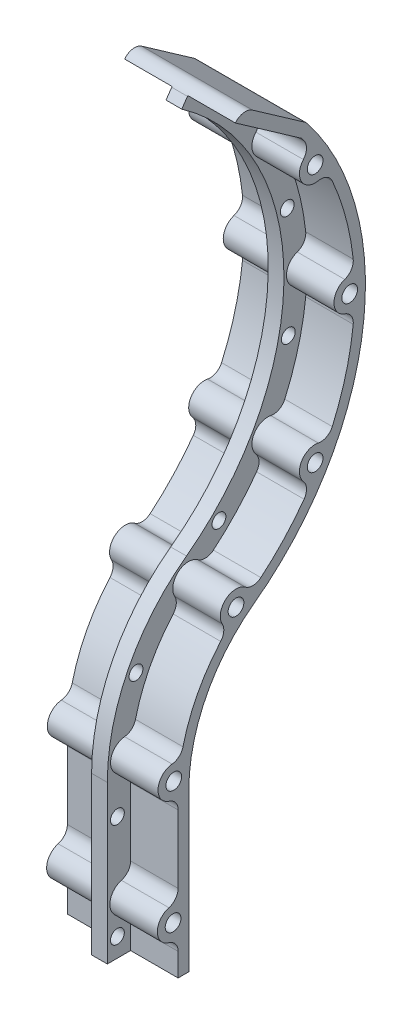
SolidWorks part; units mm, degrees
material "6061 合金"
ref_plane "前视基准面" through (0, 0, 0) normal (0, 0, 1) x (1, 0, 0)
ref_plane "上视基准面" through (0, 0, 0) normal (0, 1, 0) x (1, 0, 0)
ref_plane "右视基准面" through (0, 0, 0) normal (1, 0, 0) x (0, 0, -1)
sketch "弹链路径" plane through (0, 0, 0) normal (1, 0, 0) x (0, 0, -1)
  line L0 (0, -41.5) -> (0, 0)
  line L1 (0, 80) -> (6.1652, 79.4606)
  line L2 (0, 80) -> (3.3166, 80) construction
  arc A0 (18.3088, 36.2295) -> (0, 0) centre (45, 0) ccw
  arc A1 (18.3088, 36.2295) -> (6.1652, 79.4606) centre (4.0735, 55.5519) ccw
  dimension "D1" = 45
  dimension "D2" = 24
  dimension "D3" = 5
  dimension "D4" = 80
  dimension "D5" = 121.5
sketch "螺纹孔位" plane through (0, 0, 0) normal (1, 0, 0) x (0, 0, -1)
  line L0 (4.0735, 55.5519) -> (39.5805, 76.0519) construction
  line L1 (4.0735, 55.5519) -> (45.0735, 55.5519) construction
  line L2 (4.0735, 55.5519) -> (39.5805, 35.0519) construction
  line L3 (45, 0) -> (0, 0) construction
  line L4 (-17, -17) -> (17, -17) construction
  line L5 (0, -41.5) -> (0, 0) construction
  line L6 (-15.3402, 14.25) -> (17.1065, 2.4404) construction
  line L7 (2.9189, 45.5322) -> (27.0019, 21.4492) construction
  line L8 (45, 0) -> (27.0019, 21.4492) construction
  line L9 (45, 0) -> (17.1065, 2.4404) construction
  arc A0 (39.5805, 76.0519) -> (39.5805, 35.0519) centre (4.0735, 55.5519) cw construction
  circle A1 centre (39.5805, 76.0519) radius 1.5
  circle A2 centre (39.5805, 35.0519) radius 1.5
  circle A3 centre (45.0735, 55.5519) radius 1.5
  circle A4 centre (-17, -17) radius 1.5
  circle A5 centre (17, -17) radius 1.5
  arc A6 (-15.3402, 14.25) -> (2.9189, 45.5322) centre (45, 0) cw construction
  arc A7 (17.1065, 2.4404) -> (27.0019, 21.4492) centre (45, 0) cw construction
  circle A8 centre (-15.3402, 14.25) radius 1.5
  circle A9 centre (2.9189, 45.5322) radius 1.5
  circle A10 centre (27.0019, 21.4492) radius 1.5
  circle A11 centre (17.1065, 2.4404) radius 1.5
  point P10 (0, -17)
  dimension "D1" = 41
  dimension "D3" = 62
  dimension "D4" = 28
  dimension "D11" = 3
  dimension "D2" = 30
  dimension "D5" = 175
  dimension "D6" = 165
  dimension "D7" = 5
  dimension "D8" = 45
  dimension "D9" = 17
  dimension "D10" = 34
sketch "草图3" plane through (0, 0, 0) normal (1, 0, 0) x (0, 0, -1)
  line L0 (-19.5, 0) -> (-19.5, -25)
  line L1 (-19.5, -25) -> (-13.9, -25)
  line L2 (-13.9, -25) -> (-13.9, 0)
  line L3 (7.2554, 58.7339) -> (11.2152, 62.6937)
  line L4 (4.0735, 55.5519) -> (45.0735, 55.5519) construction
  line L5 (4.0735, 55.5519) -> (45.0735, 55.5519) construction
  line L6 (-17.6, 0) -> (-17.6, -25) construction
  line L7 (19.5, 0) -> (19.5, -25)
  line L8 (14.1, 0) -> (14.1, -25)
  line L9 (14.1, -25) -> (19.5, -25)
  line L11 (27.986, 89.7026) -> (38.1572, 82.5807)
  line L12 (27.986, 89.7026) -> (25.9267, 86.7616)
  line L13 (17.8, -25) -> (17.8, 0) construction
  line L14 (45, 0) -> (0, 0) construction
  line L15 (37.3857, 80.8013) -> (26.8962, 88.1462) construction
  line L16 (-15.5, 0) -> (-15.5, -25) construction
  line L18 (15.7, -25) -> (15.7, 0) construction
  line L19 (35.9077, 79.2727) -> (25.6917, 86.426) construction
  circle A1 centre (39.5805, 76.0519) radius 1.5 construction
  circle A2 centre (45.0735, 55.5519) radius 1.5 construction
  circle A3 centre (39.5805, 35.0519) radius 1.5 construction
  circle A4 centre (27.0019, 21.4492) radius 1.5 construction
  circle A5 centre (2.9189, 45.5322) radius 1.5 construction
  circle A6 centre (-15.3402, 14.25) radius 1.5 construction
  circle A7 centre (17.1065, 2.4404) radius 1.5 construction
  circle A8 centre (17, -17) radius 1.5 construction
  circle A9 centre (-17, -17) radius 1.5 construction
  circle A10 centre (39.5805, 76.0519) radius 1.5
  circle A11 centre (45.0735, 55.5519) radius 1.5
  circle A12 centre (39.5805, 35.0519) radius 1.5
  circle A13 centre (27.0019, 21.4492) radius 1.5
  circle A14 centre (2.9189, 45.5322) radius 1.5
  circle A15 centre (-15.3402, 14.25) radius 1.5
  circle A16 centre (17.1065, 2.4404) radius 1.5
  circle A17 centre (17, -17) radius 1.5
  circle A18 centre (-17, -17) radius 1.5
  arc A19 (10.0642, 47.4204) -> (-13.9, 0) centre (45, 0) ccw
  arc A20 (6.7426, 51.929) -> (-19.5, 0) centre (45, 0) ccw
  arc A21 (6.7426, 51.929) -> (7.2554, 58.7339) centre (4.0735, 55.5519) ccw
  arc A22 (10.0642, 47.4204) -> (11.2152, 62.6937) centre (4.0735, 55.5519) ccw
  arc A23 (7.8695, 50.3993) -> (-17.6, 0) centre (45, 0) ccw construction
  arc A24 (7.8695, 50.3993) -> (8.5989, 60.0774) centre (4.0735, 55.5519) ccw construction
  arc A25 (29.875, 20.5301) -> (19.5, 0) centre (45, 0) ccw
  arc A29 (26.672, 24.8776) -> (14.1, 0) centre (45, 0) ccw
  arc A31 (28.8666, 21.8987) -> (17.8, 0) centre (45, 0) ccw construction
  arc A32 (26.672, 24.8776) -> (25.9267, 86.7616) centre (4.0735, 55.5519) ccw
  arc A34 (28.8666, 21.8987) -> (37.3857, 80.8013) centre (4.0735, 55.5519) ccw construction
  arc A35 (29.875, 20.5301) -> (38.1572, 82.5807) centre (4.0735, 55.5519) ccw
  arc A36 (9.1151, 48.7086) -> (10.0839, 61.5623) centre (4.0735, 55.5519) ccw construction
  arc A37 (9.1151, 48.7086) -> (-15.5, 0) centre (45, 0) ccw construction
  arc A38 (27.621, 23.5894) -> (15.7, 0) centre (45, 0) ccw construction
  arc A39 (27.621, 23.5894) -> (35.9077, 79.2727) centre (4.0735, 55.5519) ccw construction
  circle A40 centre (-15.5, -22) radius 1.1
  circle A41 centre (-15.5, -2.4108) radius 1.1
  circle A42 centre (-5.8714, 32.7468) radius 1.1
  circle A43 centre (11.8184, 59.0542) radius 1.1
  circle A44 centre (15.7, -22) radius 1.1
  circle A45 centre (15.7, -5.5) radius 1.1
  circle A46 centre (18.6561, 12.8254) radius 1.1
  circle A47 centre (30.4428, 83.0992) radius 1.1 construction
  circle A48 centre (42.6935, 64.749) radius 1.1
  circle A49 centre (31.8415, 27.1789) radius 1.1
  circle A50 centre (42.866, 47.1124) radius 1.1
  point P46 (0, 80)
  dimension "D1" = 64.5
  dimension "D3" = 58.9
  dimension "D5" = 1.9
  dimension "D6" = 25.5
  dimension "D7" = 30.9
  dimension "D10" = 55
  dimension "D16" = 2.2
  dimension "D2" = 8
  dimension "D4" = 45
  dimension "D8" = 24
  dimension "D9" = 35
  dimension "D11" = 1.7
  dimension "D12" = 1.9
  dimension "D17" = 3
  dimension "D18" = 3
  dimension "D19" = 3
  dimension "D20" = 11.5
  dimension "D21" = 10.5
  dimension "D22" = 7.5
  dimension "D23" = 12.5
  dimension "D24" = 9.5
  dimension "D25" = 5.8
  dimension "D13" = 2.1
  dimension "D15" = 2.1
extrude "凸台-拉伸1" add sketch "草图3" along normal mid plane 2.5 contours L8 L9 L7 A25 A35 L11 L12 A32 A29 | A47 | A48 | A50 | A49 | A46 | A45 | A44
sketch "草图4" plane through (0, 0, 0) normal (1, 0, 0) x (0, 0, -1)
  line L2 (17.8, -25) -> (17.8, 0) construction
  line L3 (14.1, -25) -> (19.5, -25) construction
  line L10 (19.5, 0) -> (19.5, -25) construction
  line L13 (19.5, 0) -> (19.5, -25)
  line L21 (37.3857, 80.8013) -> (26.8962, 88.1462) construction
  line L22 (27.986, 89.7026) -> (38.1572, 82.5807) construction
  line L23 (27.986, 89.7026) -> (25.9267, 86.7616) construction
  line L25 (17.8, -25) -> (19.5, -25)
  line L27 (37.3857, 80.8013) -> (26.8962, 88.1462)
  line L28 (27.986, 89.7026) -> (38.1572, 82.5807)
  line L29 (27.986, 89.7026) -> (26.8962, 88.1462)
  line L30 (17.8, -25) -> (17.8, -19.3685)
  line L31 (17.8, -14.6315) -> (17.8, 0.0385)
  arc A20 (41.4094, 36.7564) -> (39.0188, 32.6159) centre (39.5805, 35.0519) ccw
  arc A21 (45.805, 57.9425) -> (45.805, 53.1614) centre (45.0735, 55.5519) ccw
  arc A31 (39.0188, 78.488) -> (41.4094, 74.3474) centre (39.5805, 76.0519) ccw
  arc A42 (17.8, -14.6315) -> (17.8, -19.3685) centre (17, -17) ccw
  arc A47 (29.875, 20.5301) -> (19.5, 0) centre (45, 0) ccw construction
  arc A48 (29.875, 20.5301) -> (38.1572, 82.5807) centre (4.0735, 55.5519) ccw construction
  arc A49 (29.875, 20.5301) -> (19.5, 0) centre (45, 0) ccw
  arc A50 (29.875, 20.5301) -> (38.1572, 82.5807) centre (4.0735, 55.5519) ccw
  arc A51 (28.8666, 21.8987) -> (37.3857, 80.8013) centre (4.0735, 55.5519) ccw construction
  arc A52 (28.8666, 21.8987) -> (17.8, 0) centre (45, 0) ccw construction
  arc A53 (29.3633, 22.2703) -> (39.0188, 32.6159) centre (4.0735, 55.5519) ccw
  arc A54 (25.7939, 19.2605) -> (18.2066, 4.6853) centre (45, 0) ccw
  arc A55 (18.2066, 4.6853) -> (17.8, 0.0385) centre (17.1065, 2.4404) ccw
  arc A56 (29.3633, 22.2703) -> (25.7939, 19.2605) centre (27.0019, 21.4492) ccw
  arc A57 (41.4094, 36.7564) -> (45.805, 53.1614) centre (4.0735, 55.5519) ccw
  arc A58 (45.805, 57.9425) -> (41.4094, 74.3474) centre (4.0735, 55.5519) ccw
  arc A59 (39.0188, 78.488) -> (37.3857, 80.8013) centre (4.0735, 55.5519) ccw
  dimension "D1" = 2.5
extrude "凸台-拉伸2" add sketch "草图4" along normal mid plane 17.6
sketch "草图5" plane through (8.8, 0, 0) normal (1, 0, 0) x (0, 0, -1)
  point P0 (39.5805, 76.0519)
  point P1 (45.0735, 55.5519)
  point P3 (39.5805, 35.0519)
  point P5 (27.0019, 21.4492)
  point P7 (17.1065, 2.4404)
  point P9 (17, -17)
hole_wizard "M3 螺纹孔1" positions "草图5" profile "草图6" tap size "M3" standard "GB" end condition through all
sketch "草图6" plane through (8.8, 76.0519, -39.5805) normal (0, 1, 0) x (0, 0, -1)
  line L0 (0, 0) -> (0, 17.6)
  line L1 (0, 17.6) -> (1.25, 17.6)
  line L2 (1.25, 17.6) -> (1.25, 0)
  line L5 (1.25, 0) -> (0, 0)
  line L11 (0, -6.35) -> (0, 107.95) construction
  dimension "通孔螺纹孔钻头直径" = 2.5
  dimension "通孔螺纹孔钻头深度" = 17.6
cosmetic thread "孔螺纹线1" parameters "D2"=3
cosmetic thread "孔螺纹线2" parameters "D2"=3
cosmetic thread "孔螺纹线3" parameters "D2"=3
cosmetic thread "孔螺纹线4" parameters "D2"=3
cosmetic thread "孔螺纹线5" parameters "D2"=3
cosmetic thread "孔螺纹线6" parameters "D2"=3
fillet "R2 圆角1" radius 2 26 edges at (0, 82.5807, -38.1572) (0, 89.7026, -27.986) (5.025, -19.3685, -17.8) (-5.025, -19.3685, -17.8) (-5.025, -14.6315, -17.8) (5.025, -14.6315, -17.8) (5.025, 0.0385, -17.8) (-5.025, 0.0385, -17.8) (-5.025, 4.6853, -18.2066) (5.025, 4.6853, -18.2066) (-5.025, 19.2605, -25.7939) (5.025, 19.2605, -25.7939) (-5.025, 22.2703, -29.3633) (5.025, 22.2703, -29.3633) (-5.025, 32.6159, -39.0188) (5.025, 32.6159, -39.0188) (-5.025, 36.7564, -41.4094) (5.025, 36.7564, -41.4094) (-5.025, 53.1614, -45.805) (5.025, 53.1614, -45.805) (5.025, 57.9425, -45.805) (-5.025, 57.9425, -45.805) (5.025, 74.3474, -41.4094) (-5.025, 74.3474, -41.4094) (-5.025, 78.488, -39.0188) (5.025, 78.488, -39.0188)
